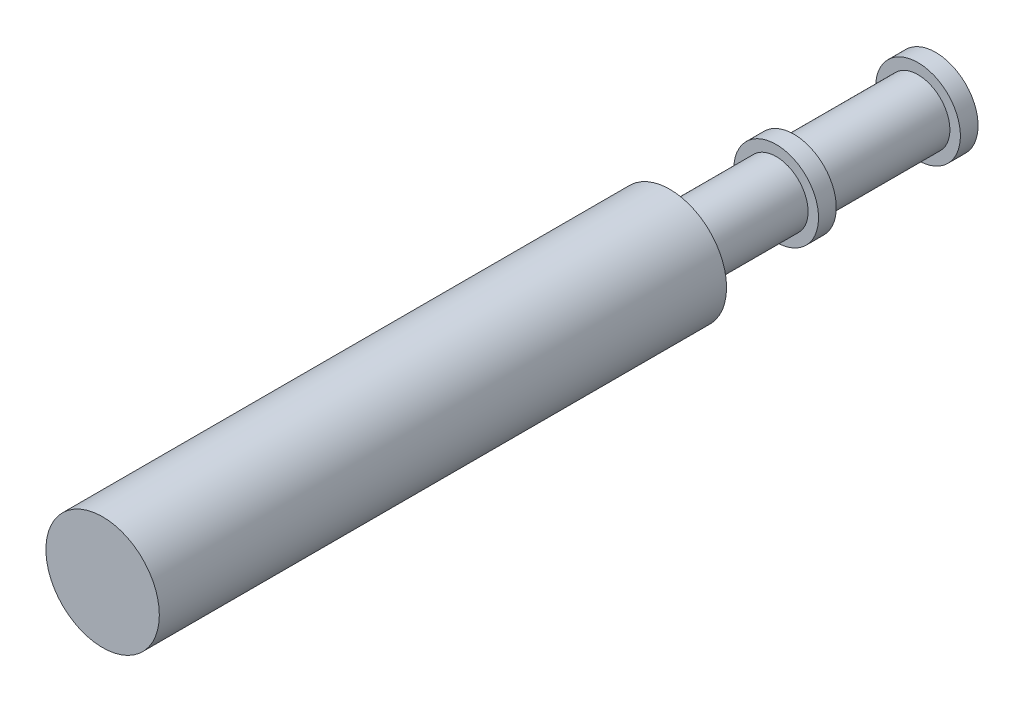
from build123d import *

# Parameters (mm, degrees)
SKETCH5_R           = 16
BOSS_EXTRUDE1_DEPTH = 60
SKETCH6_R           = 9
BOSS_EXTRUDE2_DEPTH = 70
BOSS_EXTRUDE3_START = 100
SKETCH7_R           = 16
BOSS_EXTRUDE3_DEPTH = 100
SKETCH8_R           = 11.952224842
BOSS_EXTRUDE4_DEPTH = 5
LPATTERN1_COUNT     = 2
LPATTERN1_PITCH     = 40


with BuildPart() as part:
    # Sketch5 → Boss-Extrude1 (new body)
    with BuildSketch(Plane.XY):
        with Locations((-19.20096517, 5.868531988)):
            Circle(SKETCH5_R)
    extrude(amount=-BOSS_EXTRUDE1_DEPTH)

    # Sketch6 → Boss-Extrude2 (add)
    with BuildSketch(Plane(origin=(0, 0, -60), x_dir=(-1, 0, 0), z_dir=(0, 0, -1))):
        with Locations((19.20096517, 5.868531988)):
            Circle(SKETCH6_R)
    extrude(amount=BOSS_EXTRUDE2_DEPTH)

    # Sketch7 → Boss-Extrude3 (add)
    with BuildSketch(Plane.XY.offset(BOSS_EXTRUDE3_START)):
        with Locations((-19.20096517, 5.868531988)):
            Circle(SKETCH7_R)
    extrude(amount=-BOSS_EXTRUDE3_DEPTH)

    # Sketch8 → Boss-Extrude4 (add)
    with BuildSketch(Plane(origin=(0, 0, -130), x_dir=(-1, 0, 0), z_dir=(0, 0, -1))):
        with Locations((19.20096517, 5.868531988)):
            Circle(SKETCH8_R)
    boss_extrude4 = extrude(amount=BOSS_EXTRUDE4_DEPTH)

    # LPattern1: Boss-Extrude4 ×2
    with Locations(*[(0, 0, i * LPATTERN1_PITCH) for i in range(1, LPATTERN1_COUNT)]):
        add(boss_extrude4)


solid = part.part
